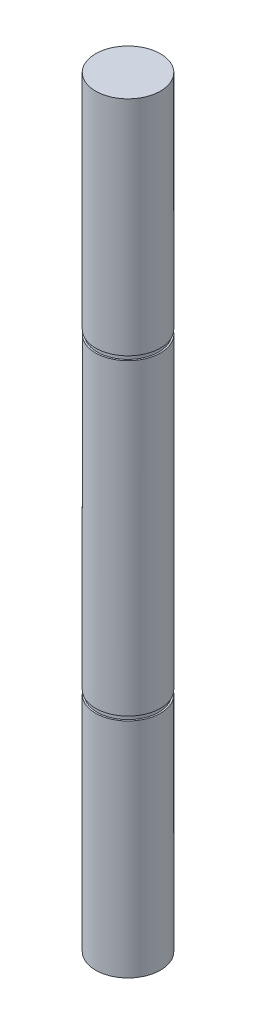
from build123d import *

# Parameters (mm, degrees)
SKETCH_1_R          = 10
EXTRUDE_1_DEPTH     = 235
CUT_EXTRUDE_START   = 1.3
SKETCH_7_R          = 10
SKETCH_7_R_2        = 9.5
CUT_EXTRUDE_3_DEPTH = 1.3
SKETCH_8_R          = 10
SKETCH_8_R_2        = 9.5
CUT_EXTRUDE_4_DEPTH = 1.3
ZJCQC_DEPTH         = 3.5


with BuildPart() as part:
    # 草图1 → 凸台-拉伸1 (new body)
    with BuildSketch(Plane(origin=(0, 0, 0), x_dir=(1, 0, 0), z_dir=(0, 1, 0))):
        with Locations(Location((0, 0, 0), (0, 0, 90))):
            Circle(SKETCH_1_R)
    extrude(amount=EXTRUDE_1_DEPTH)

    # 草图7 → 切除-拉伸3 (cut)
    with BuildSketch(Plane(origin=(0, 70, 0), x_dir=(-1, 0, 0), z_dir=(0, -1, 0)).offset(CUT_EXTRUDE_START)):
        with Locations(Location((0, 0, 0), (0, 0, 90))):
            Circle(SKETCH_7_R)
        with Locations(Location((0, 0, 0), (0, 0, 90))):
            Circle(SKETCH_7_R_2, mode=Mode.SUBTRACT)
    extrude(amount=-CUT_EXTRUDE_3_DEPTH, mode=Mode.SUBTRACT)

    # 草图8 → 切除-拉伸4 (cut)
    with BuildSketch(Plane(origin=(0, 165, 0), x_dir=(1, 0, 0), z_dir=(0, 1, 0))):
        with Locations(Location((0, 0, 0), (0, 0, 90))):
            Circle(SKETCH_8_R)
        with Locations(Location((0, 0, 0), (0, 0, 90))):
            Circle(SKETCH_8_R_2, mode=Mode.SUBTRACT)
    extrude(amount=CUT_EXTRUDE_4_DEPTH, mode=Mode.SUBTRACT)

    # MyToolsZJC → ZJCQC (cut)
    with BuildSketch(Plane.YX.offset(10)):
        with BuildLine():
            Line((115.5, 3), (119.5, 3))
            ThreePointArc((119.5, 3), (122.5, 0), (119.5, -3))
            Line((119.5, -3), (115.5, -3))
            ThreePointArc((115.5, -3), (112.5, 0), (115.5, 3))
        make_face()
    extrude(amount=-ZJCQC_DEPTH, mode=Mode.SUBTRACT)


solid = part.part
